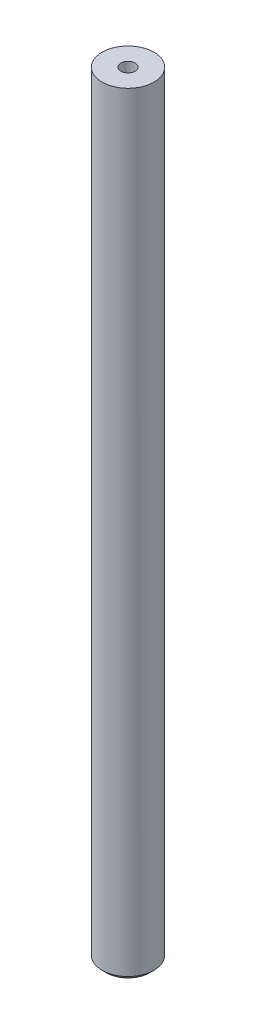
from build123d import *

# Parameters (mm, degrees)
SKETCH1_R             = 6
BOSS_EXTRUDE1_DEPTH   = 179
M4_TAPPED_HOLE1_D     = 3.3
M4_TAPPED_HOLE1_DEPTH = 30
M4_TAPPED_HOLE1_TIP   = 0.991420021
CHAMFER1_SIZE         = 1


with BuildPart() as part:
    # Sketch1 → Boss-Extrude1 (new body)
    with BuildSketch(Plane(origin=(0, 0, 0), x_dir=(1, 0, 0), z_dir=(0, 1, 0))):
        with Locations(Location((0, 0, 0), (0, 0, 90))):
            Circle(SKETCH1_R)
    extrude(amount=BOSS_EXTRUDE1_DEPTH)

    # M4 Tapped Hole1
    with Locations(Plane(origin=(0, 179, 0), x_dir=(1, 0, 0), z_dir=(0, 1, 0))):
        with Locations((0, 0), (-123.257585015, 97.244885399), (-195.107309259, 6.175586916), (-71.849724244, -91.069298483)):
            Hole(M4_TAPPED_HOLE1_D / 2, depth=M4_TAPPED_HOLE1_DEPTH)
            with Locations((0, 0, -(M4_TAPPED_HOLE1_DEPTH + M4_TAPPED_HOLE1_TIP / 2))):  # 118° drill point
                Cone(0, M4_TAPPED_HOLE1_D / 2, M4_TAPPED_HOLE1_TIP, mode=Mode.SUBTRACT)

    # Chamfer1
    chamfer1_edges = [part.edges().sort_by_distance(p)[0] for p in [
        (0, 0, 6),
    ]]
    chamfer(chamfer1_edges, length=CHAMFER1_SIZE)


solid = part.part
